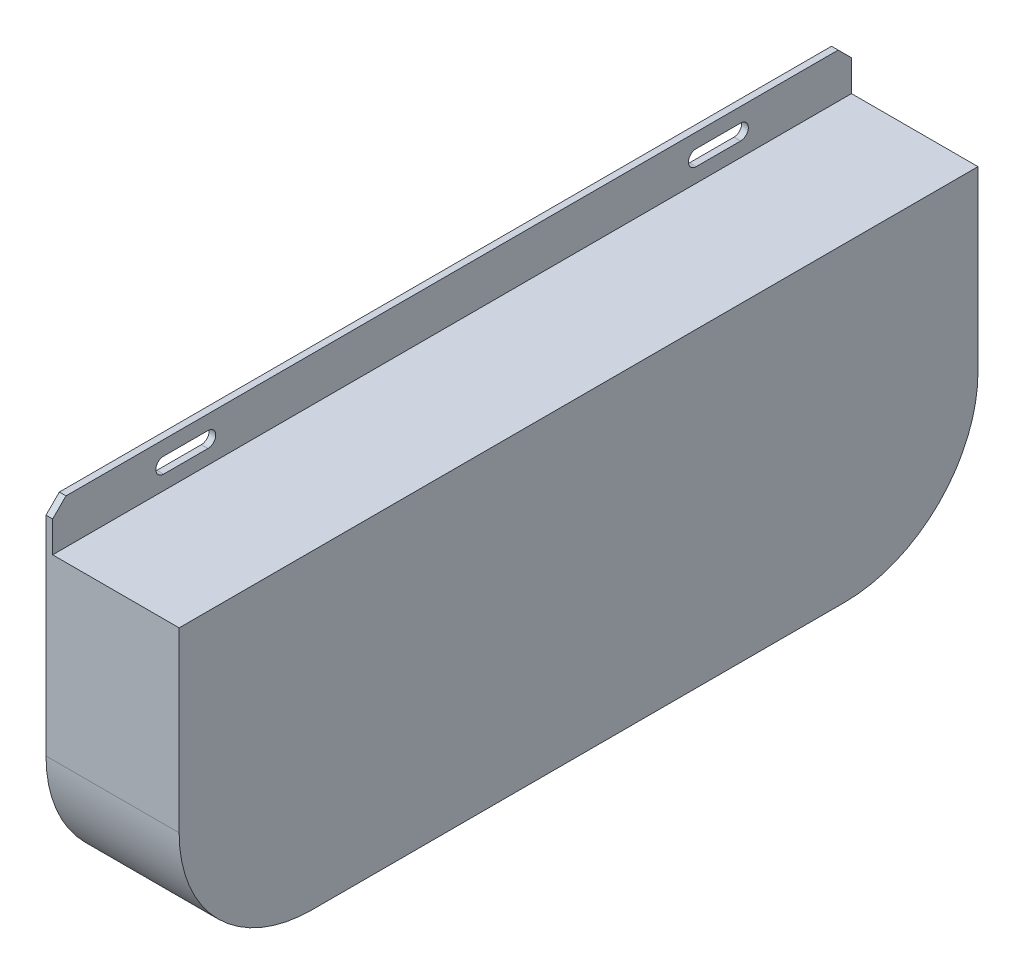
from build123d import *

# Parameters (mm, degrees)
EXTRUDE_1_DEPTH     = 30
SHELL_1_T           = -1.5
SKETCH_2_W          = 1.5
SKETCH_2_H          = 180
EXTRUDE_2_DEPTH     = 10
SKETCH_5_W          = 1.5
SKETCH_5_H          = 20
EXTRUDE_3_DEPTH     = 10
CUT_EXTRUDE_2_DEPTH = 148.786263339
CHAMFER_1_SIZE      = 3
CHAMFER_2_SIZE      = 3


with BuildPart() as part:
    # 草图1 → 凸台-拉伸1 (new body)
    with BuildSketch(Plane(origin=(0, 0, 0), x_dir=(0, 0, -1), z_dir=(1, 0, 0))):
        with BuildLine():
            Line((-54.319308007, 7.661260091), (125.680691993, 7.661260091))
            Line((125.680691993, 7.661260091), (125.680691993, -32.338739909))
            ThreePointArc((125.680691993, -32.338739909), (116.893895429, -53.551943345), (95.680691993, -62.338739909))
            Line((95.680691993, -62.338739909), (-24.319308007, -62.338739909))
            ThreePointArc((-24.319308007, -62.338739909), (-45.532511442, -53.551943345), (-54.319308007, -32.338739909))
            Line((-54.319308007, -32.338739909), (-54.319308007, 7.661260091))
        make_face()
    extrude(amount=EXTRUDE_1_DEPTH)

    # 抽壳1
    shell_1_openings = [part.faces().sort_by_distance(p)[0] for p in [
        (0, -26.44372844, -35.680691993),
    ]]
    offset(amount=SHELL_1_T, openings=shell_1_openings, kind=Kind.INTERSECTION)

    # 草图2 → 凸台-拉伸2 (add)
    with BuildSketch(Plane(origin=(0, 7.661260091, 0), x_dir=(1, 0, 0), z_dir=(0, 1, 0))):
        with Locations((0.75, 35.680691993)):
            Rectangle(SKETCH_2_W, SKETCH_2_H)
    extrude(amount=EXTRUDE_2_DEPTH)

    # 草图5 → 凸台-拉伸3 (add)
    with BuildSketch(Plane.XZ.offset(62.338739909)):
        with Locations((0.75, -35.680691993)):
            Rectangle(SKETCH_5_W, SKETCH_5_H)
    extrude(amount=EXTRUDE_3_DEPTH)

    # 草图4 → 切除-拉伸2 (cut, through all)
    with BuildSketch(Plane(origin=(1.5, 0, 0), x_dir=(0, 0, -1), z_dir=(1, 0, 0))):
        with BuildLine():
            Line((-29.319308007, 14.411260091), (-19.319308007, 14.411260091))
            ThreePointArc((-19.319308007, 14.411260091), (-17.569308007, 12.661260091), (-19.319308007, 10.911260091))
            Line((-19.319308007, 10.911260091), (-29.319308007, 10.911260091))
            ThreePointArc((-29.319308007, 10.911260091), (-31.069308007, 12.661260091), (-29.319308007, 14.411260091))
        make_face()
        with BuildLine():
            Line((90.680691993, 14.411260091), (100.680691993, 14.411260091))
            ThreePointArc((100.680691993, 14.411260091), (102.430691993, 12.661260091), (100.680691993, 10.911260091))
            Line((100.680691993, 10.911260091), (90.680691993, 10.911260091))
            ThreePointArc((90.680691993, 10.911260091), (88.930691993, 12.661260091), (90.680691993, 14.411260091))
        make_face()
        with BuildLine():
            Line((30.680691993, -65.588739909), (40.680691993, -65.588739909))
            ThreePointArc((40.680691993, -65.588739909), (42.430691993, -67.338739909), (40.680691993, -69.088739909))
            Line((40.680691993, -69.088739909), (30.680691993, -69.088739909))
            ThreePointArc((30.680691993, -69.088739909), (28.930691993, -67.338739909), (30.680691993, -65.588739909))
        make_face()
    extrude(amount=-CUT_EXTRUDE_2_DEPTH, mode=Mode.SUBTRACT)

    # 倒角1
    chamfer_1_edges = [part.edges().sort_by_distance(p)[0] for p in [
        (0.75, 17.661260091, -125.680691993),
        (0.75, 17.661260091, 54.319308007),
    ]]
    chamfer(chamfer_1_edges, length=CHAMFER_1_SIZE)

    # 倒角2
    chamfer_2_edges = [part.edges().sort_by_distance(p)[0] for p in [
        (0.75, -72.338739909, -45.680691993),
        (0.75, -72.338739909, -25.680691993),
    ]]
    chamfer(chamfer_2_edges, length=CHAMFER_2_SIZE)


solid = part.part
